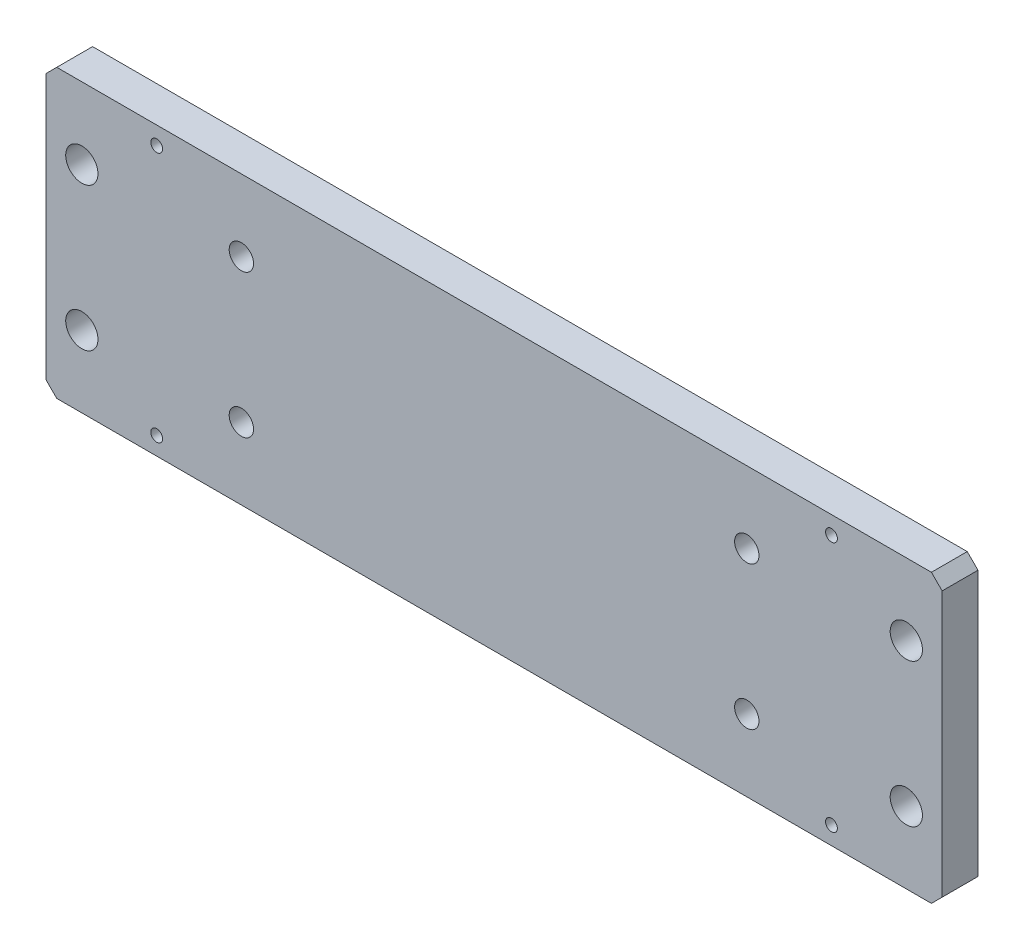
from build123d import *

# Parameters (mm, degrees)
SKETCH_1_W            = 250
SKETCH_1_H            = 80
EXTRUDE_1_DEPTH       = 10
HOLE_WIZARD_9_0_9_1_D = 9
CHAMFER_1_SIZE        = 3
HOLE_WIZARD_M8_1_D    = 6.8
HOLE_WIZARD_M4_1_D    = 3.3


with BuildPart() as part:
    # 草图1 → 凸台-拉伸1 (new body)
    with BuildSketch(Plane.XY):
        with Locations((0, 40)):
            Rectangle(SKETCH_1_W, SKETCH_1_H)
    extrude(amount=EXTRUDE_1_DEPTH)

    # Ø9.0 (9) 直径孔1 (through all)
    with Locations(Plane.XY.offset(10)):
        with Locations((115, 20), (115, 60)):
            hole_wizard_9_0_9_1 = Hole(HOLE_WIZARD_9_0_9_1_D / 2)

    # 镜向1: Ø9.0 (9) 直径孔1 across plane
    add(hole_wizard_9_0_9_1.mirror(Plane(origin=(0, 0, 0), x_dir=(0, 0, 1), z_dir=(1, 0, 0))), mode=Mode.SUBTRACT)

    # 倒角1
    chamfer_1_edges = [part.edges().sort_by_distance(p)[0] for p in [
        (-125, 80, 5),
        (125, 80, 5),
        (125, 0, 5),
        (-125, 0, 5),
    ]]
    chamfer(chamfer_1_edges, length=CHAMFER_1_SIZE)

    # M8 螺纹孔1 (through all)
    with Locations(Plane.XY.offset(10)):
        with Locations((70.5, 60), (70.5, 20)):
            hole_wizard_m8_1 = Hole(HOLE_WIZARD_M8_1_D / 2)

    # 镜向2: M8 螺纹孔1 across plane
    add(hole_wizard_m8_1.mirror(Plane(origin=(0, 0, 0), x_dir=(0, 0, 1), z_dir=(1, 0, 0))), mode=Mode.SUBTRACT)

    # M4 螺纹孔1 (through all)
    with Locations(Plane.XY.offset(10)):
        with Locations((-94.121851999, 75), (-94.121851999, 5)):
            hole_wizard_m4_1 = Hole(HOLE_WIZARD_M4_1_D / 2)

    # 镜向3: M4 螺纹孔1 across plane
    add(hole_wizard_m4_1.mirror(Plane.ZY), mode=Mode.SUBTRACT)


solid = part.part
